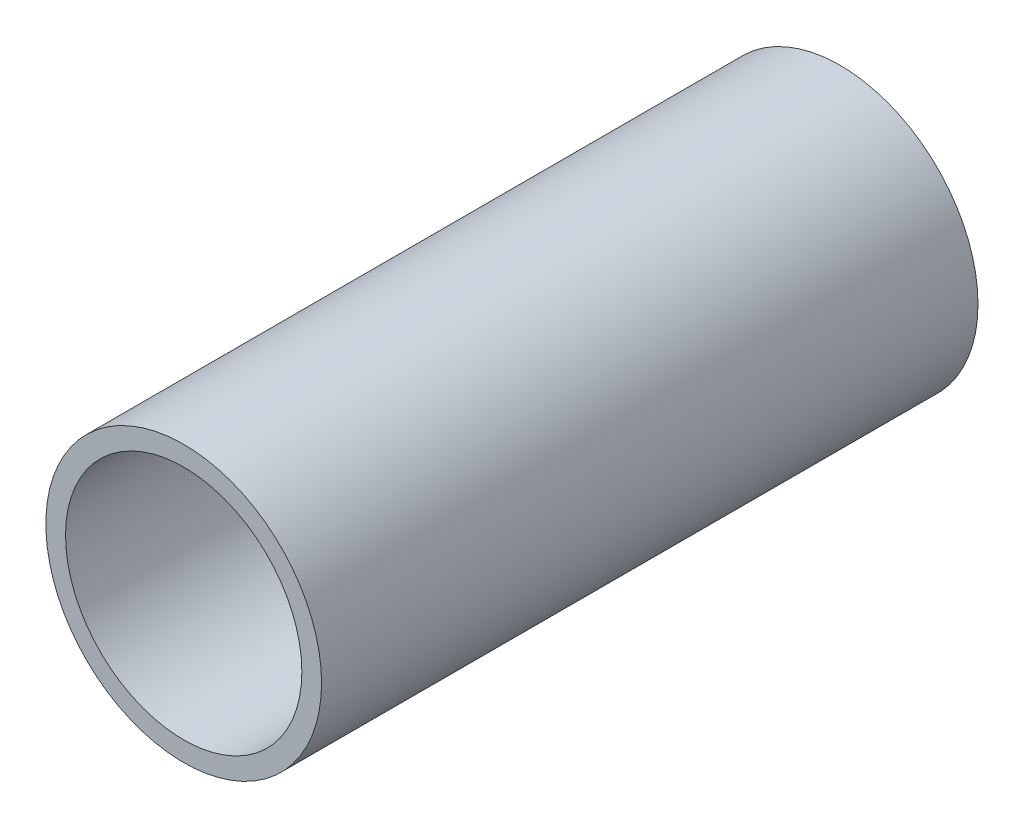
from build123d import *

# Parameters (mm, degrees)
SKETCH_1_R           = 21
SKETCH_1_R_2         = 18
BOSS_EXTRUDE_1_DEPTH = 100


with BuildPart() as part:
    # Sketch 1 → Boss-Extrude 1 (new body)
    with BuildSketch(Plane.XY):
        Circle(SKETCH_1_R)
        Circle(SKETCH_1_R_2, mode=Mode.SUBTRACT)
    extrude(amount=BOSS_EXTRUDE_1_DEPTH)


solid = part.part
